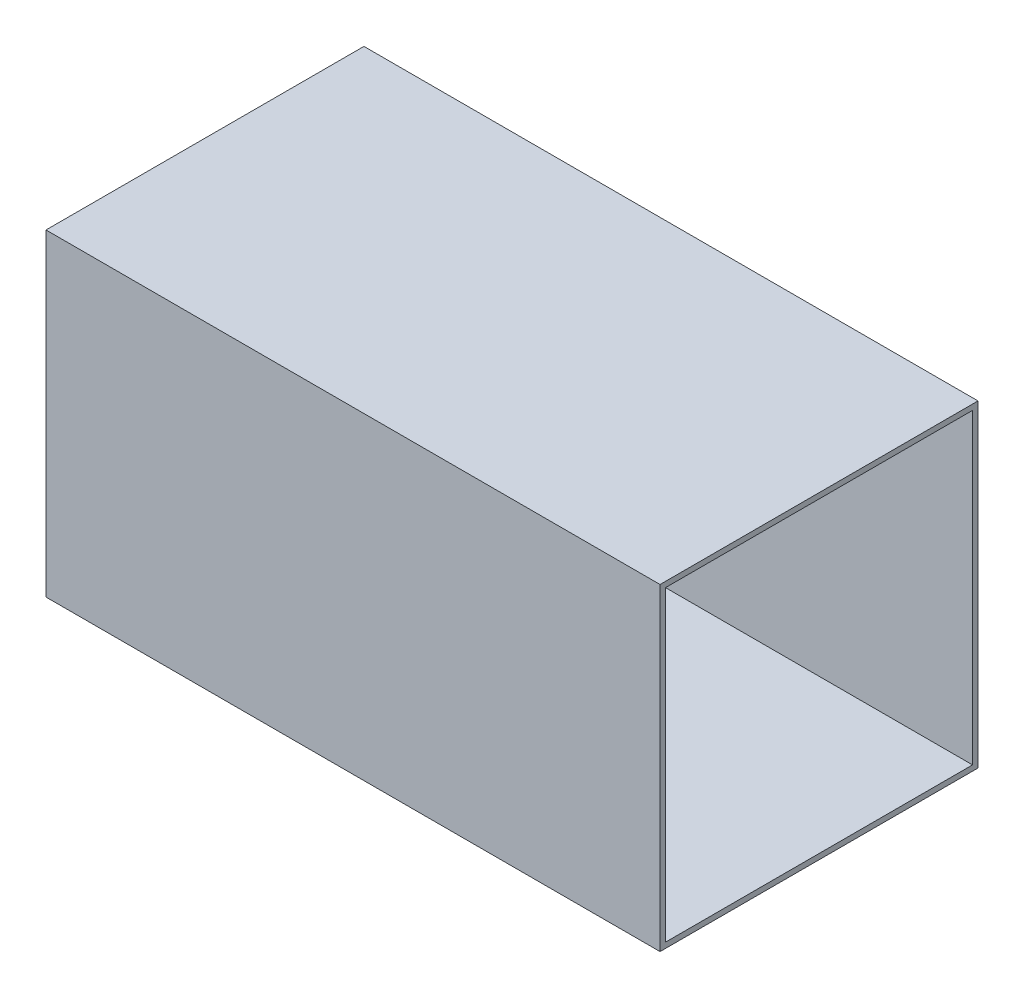
SolidWorks part; units mm, degrees
ref_plane "Front Plane" through (0, 0, 0) normal (0, 0, 1) x (1, 0, 0)
ref_plane "Top Plane" through (0, 0, 0) normal (0, 1, 0) x (1, 0, 0)
ref_plane "Right Plane" through (0, 0, 0) normal (1, 0, 0) x (0, 0, -1)
other "Configuration Table"
sketch "Sketch1" plane through (0, 0, 0) normal (1, 0, 0) x (0, 0, -1)
  line L1 (-225, 225) -> (225, 225)
  line L2 (-225, 225) -> (-225, -225)
  line L3 (-225, -225) -> (225, -225)
  line L4 (225, 225) -> (225, -225)
  line L5 (-225, 225) -> (225, -225) construction
  line L6 (-225, -225) -> (225, 225) construction
  line L7 (-233, 233) -> (233, 233)
  line L8 (-233, 233) -> (-233, -233)
  line L9 (-233, -233) -> (233, -233)
  line L10 (233, 233) -> (233, -233)
  line L11 (-233, 233) -> (233, -233) construction
  line L12 (-233, -233) -> (233, 233) construction
  point P0 (0, 0)
  point P6 (0, 0)
  dimension "D1" = 450
  dimension "D2" = 450
  dimension "D3" = 466
  dimension "D4" = 466
extrude "Boss-Extrude1" add sketch "Sketch1" along normal blind 900
